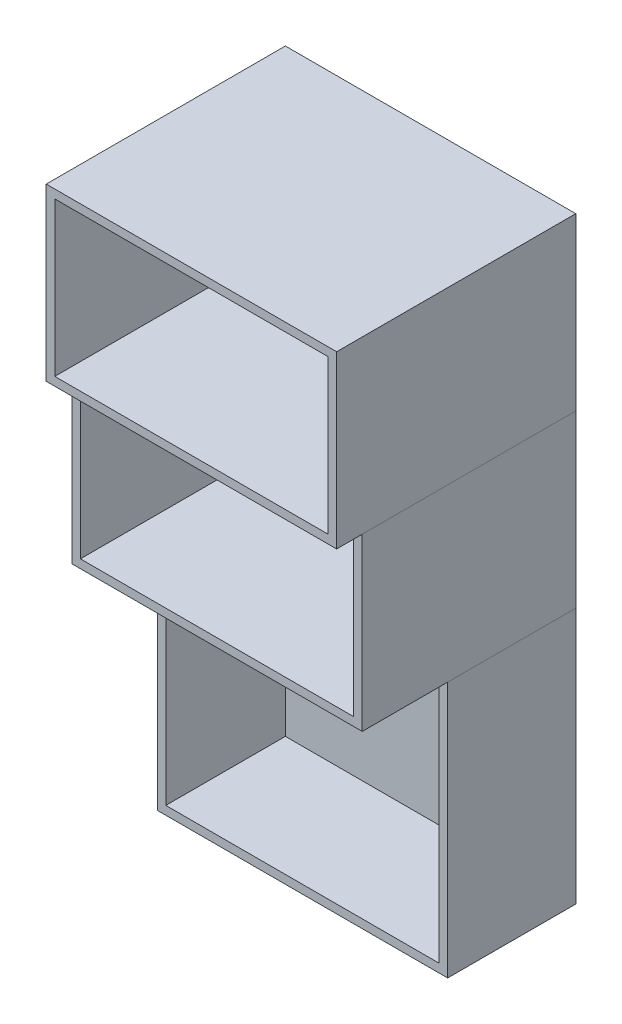
SolidWorks part; units mm, degrees
ref_plane "前视基准面" through (0, 0, 0) normal (0, 0, 1) x (1, 0, 0)
ref_plane "上视基准面" through (0, 0, 0) normal (0, 1, 0) x (1, 0, 0)
ref_plane "右视基准面" through (0, 0, 0) normal (1, 0, 0) x (0, 0, -1)
sketch "草图1" plane through (0, 0, 0) normal (0, 0, 1) x (1, 0, 0)
  line L1 (-170, -100) -> (170, -100)
  line L2 (-170, -100) -> (-170, 100)
  line L3 (-170, 100) -> (170, 100)
  line L4 (170, -100) -> (170, 100)
  line L5 (-170, -100) -> (170, 100) construction
  line L6 (-170, 100) -> (170, -100) construction
  point P0 (0, 0)
  dimension "D1" = 340
  dimension "D2" = 200
extrude "凸台-拉伸1" add sketch "草图1" along normal blind 280
shell "抽壳1" thickness 10
sketch "草图2" plane through (0, 0, 0) normal (0, 0, -1) x (-1, 0, 0)
  line L0 (170, 100) -> (170, -100) construction
  line L1 (-170, -100) -> (170, -100)
  line L2 (-170, -100) -> (-170, -300)
  line L3 (-170, -300) -> (170, -300)
  line L4 (170, -100) -> (170, -300)
  dimension "D1" = 200
extrude "凸台-拉伸2" add sketch "草图2" against normal blind 250 separate body
shell "抽壳2" thickness 10
sketch "草图3" plane through (0, 0, 0) normal (0, 0, -1) x (-1, 0, 0)
  line L0 (170, -300) -> (170, -100) construction
  line L1 (-170, -300) -> (170, -300)
  line L2 (-170, -300) -> (-170, -600)
  line L3 (-170, -600) -> (170, -600)
  line L4 (170, -300) -> (170, -600)
  dimension "D1" = 300
extrude "凸台-拉伸3" add sketch "草图3" against normal blind 150 separate body
shell "抽壳3" thickness 10
